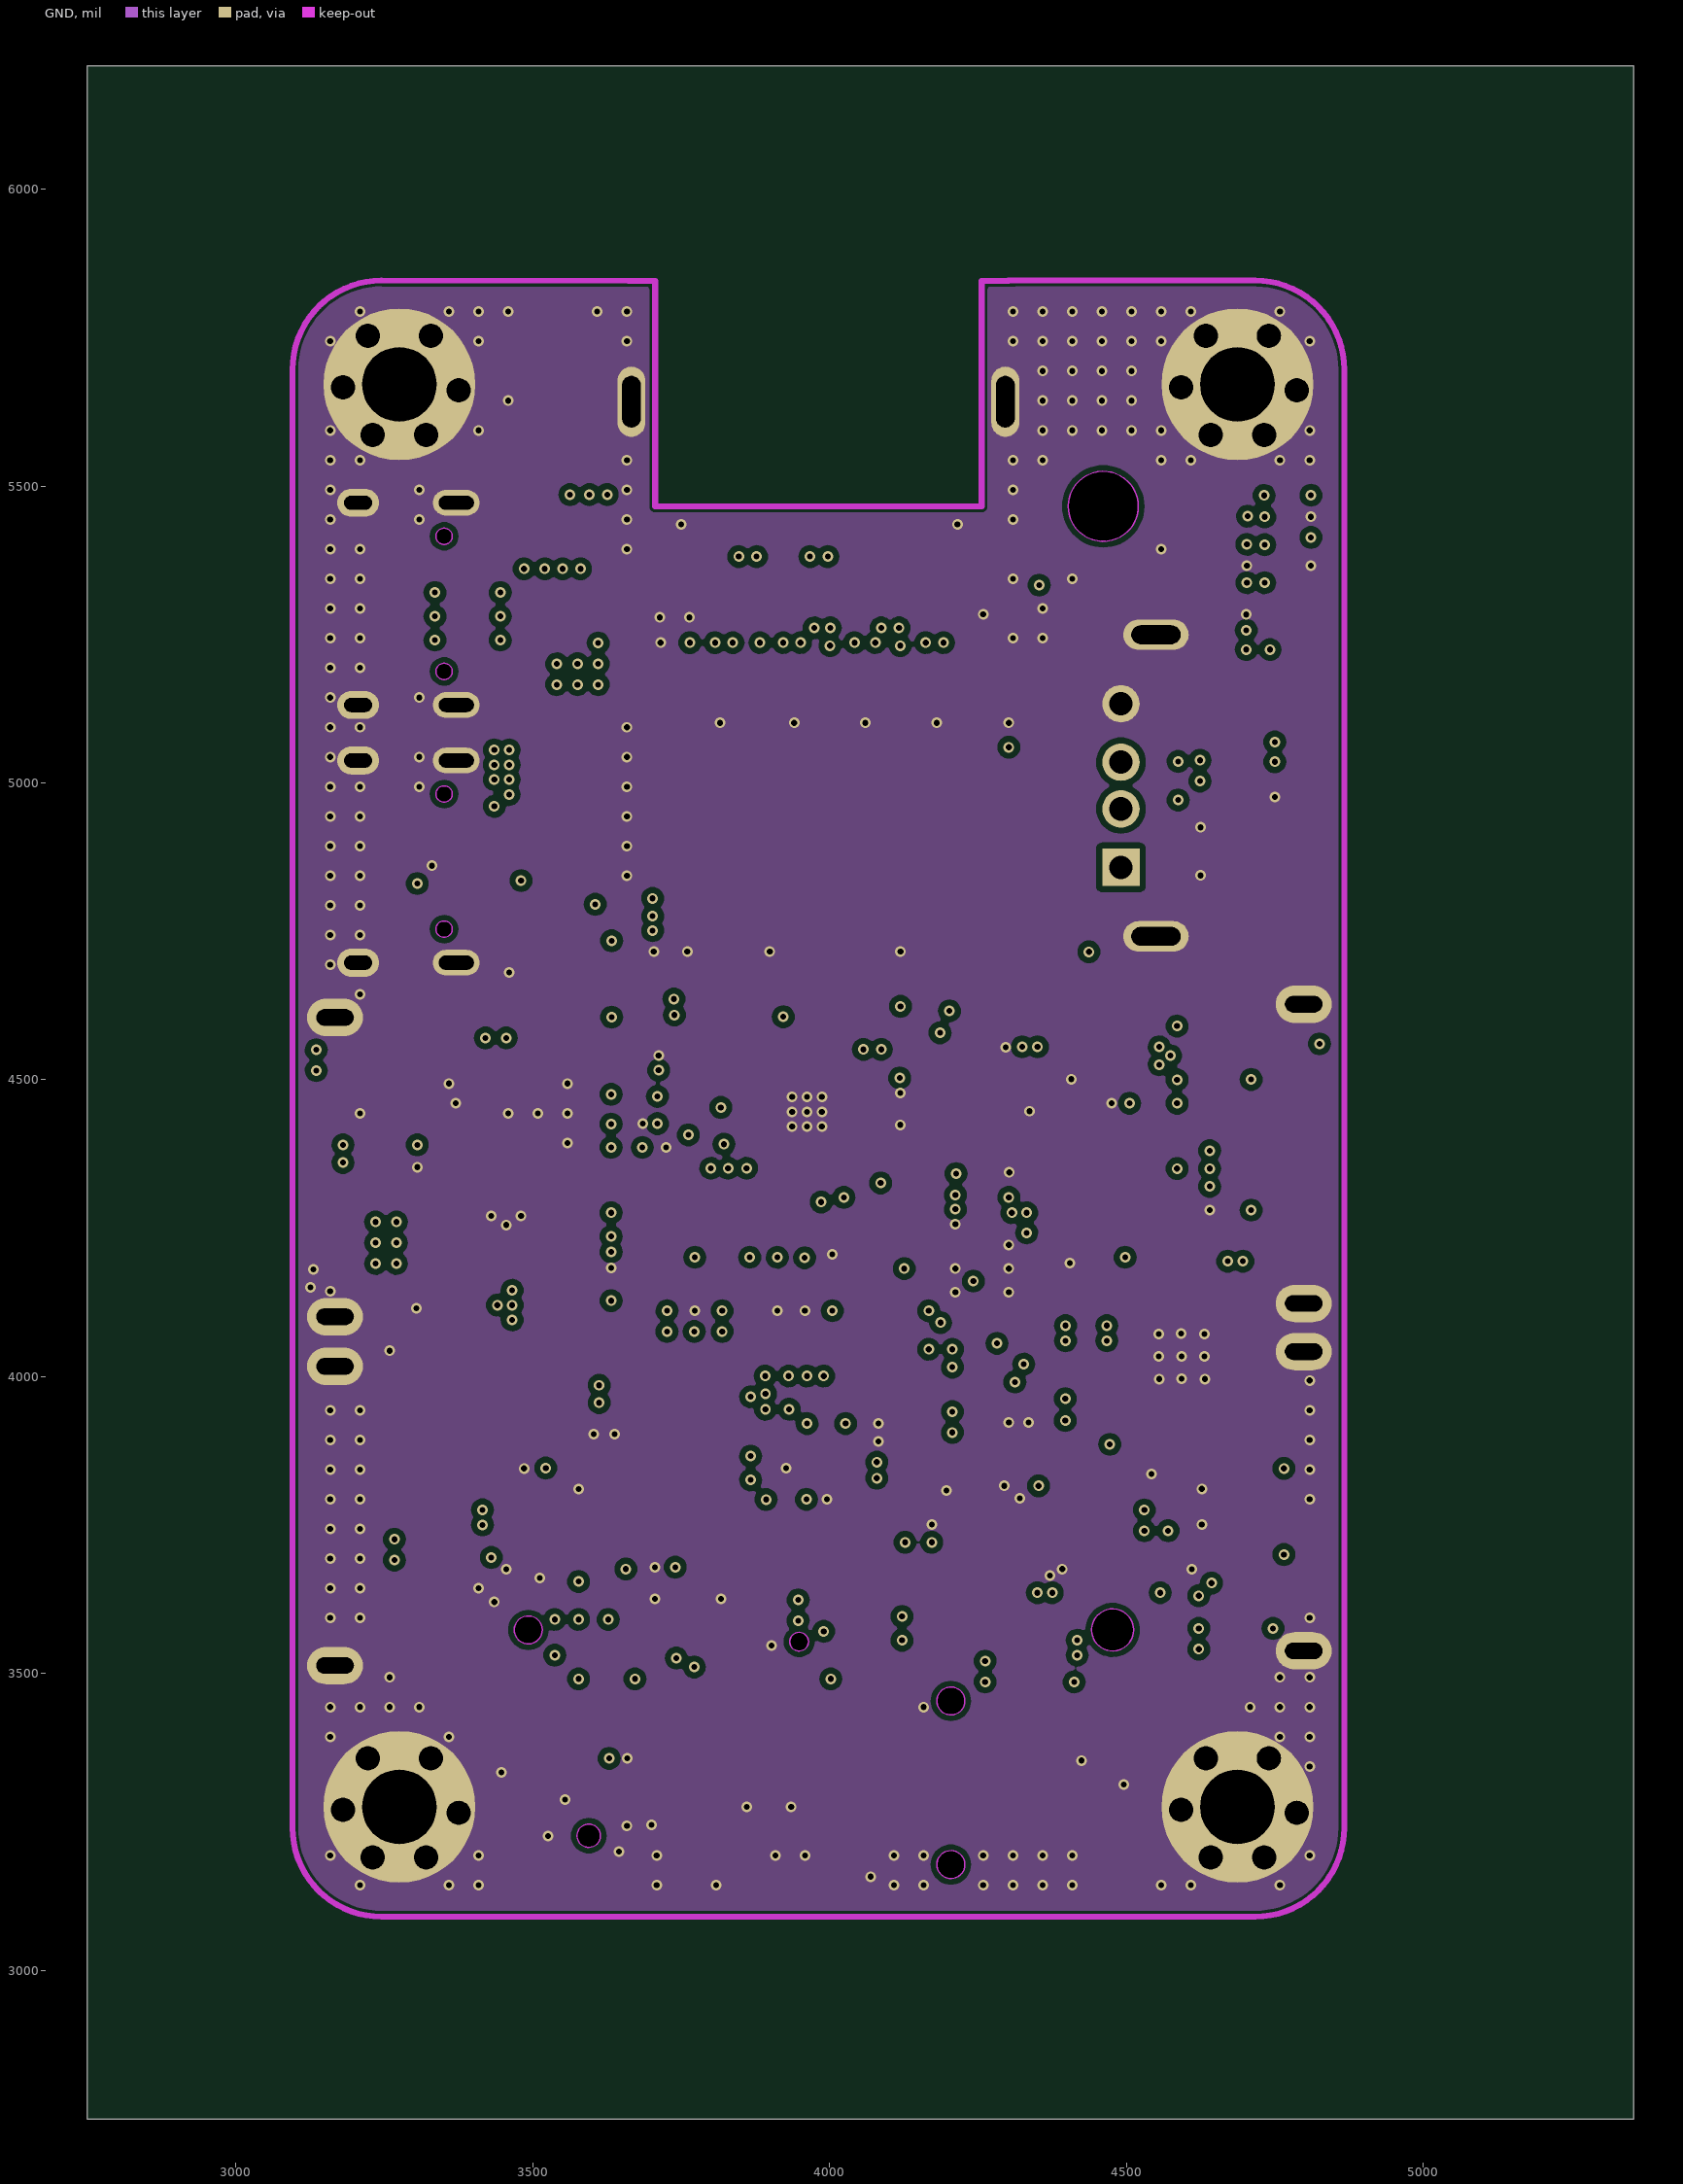
[diagram p0: GND]
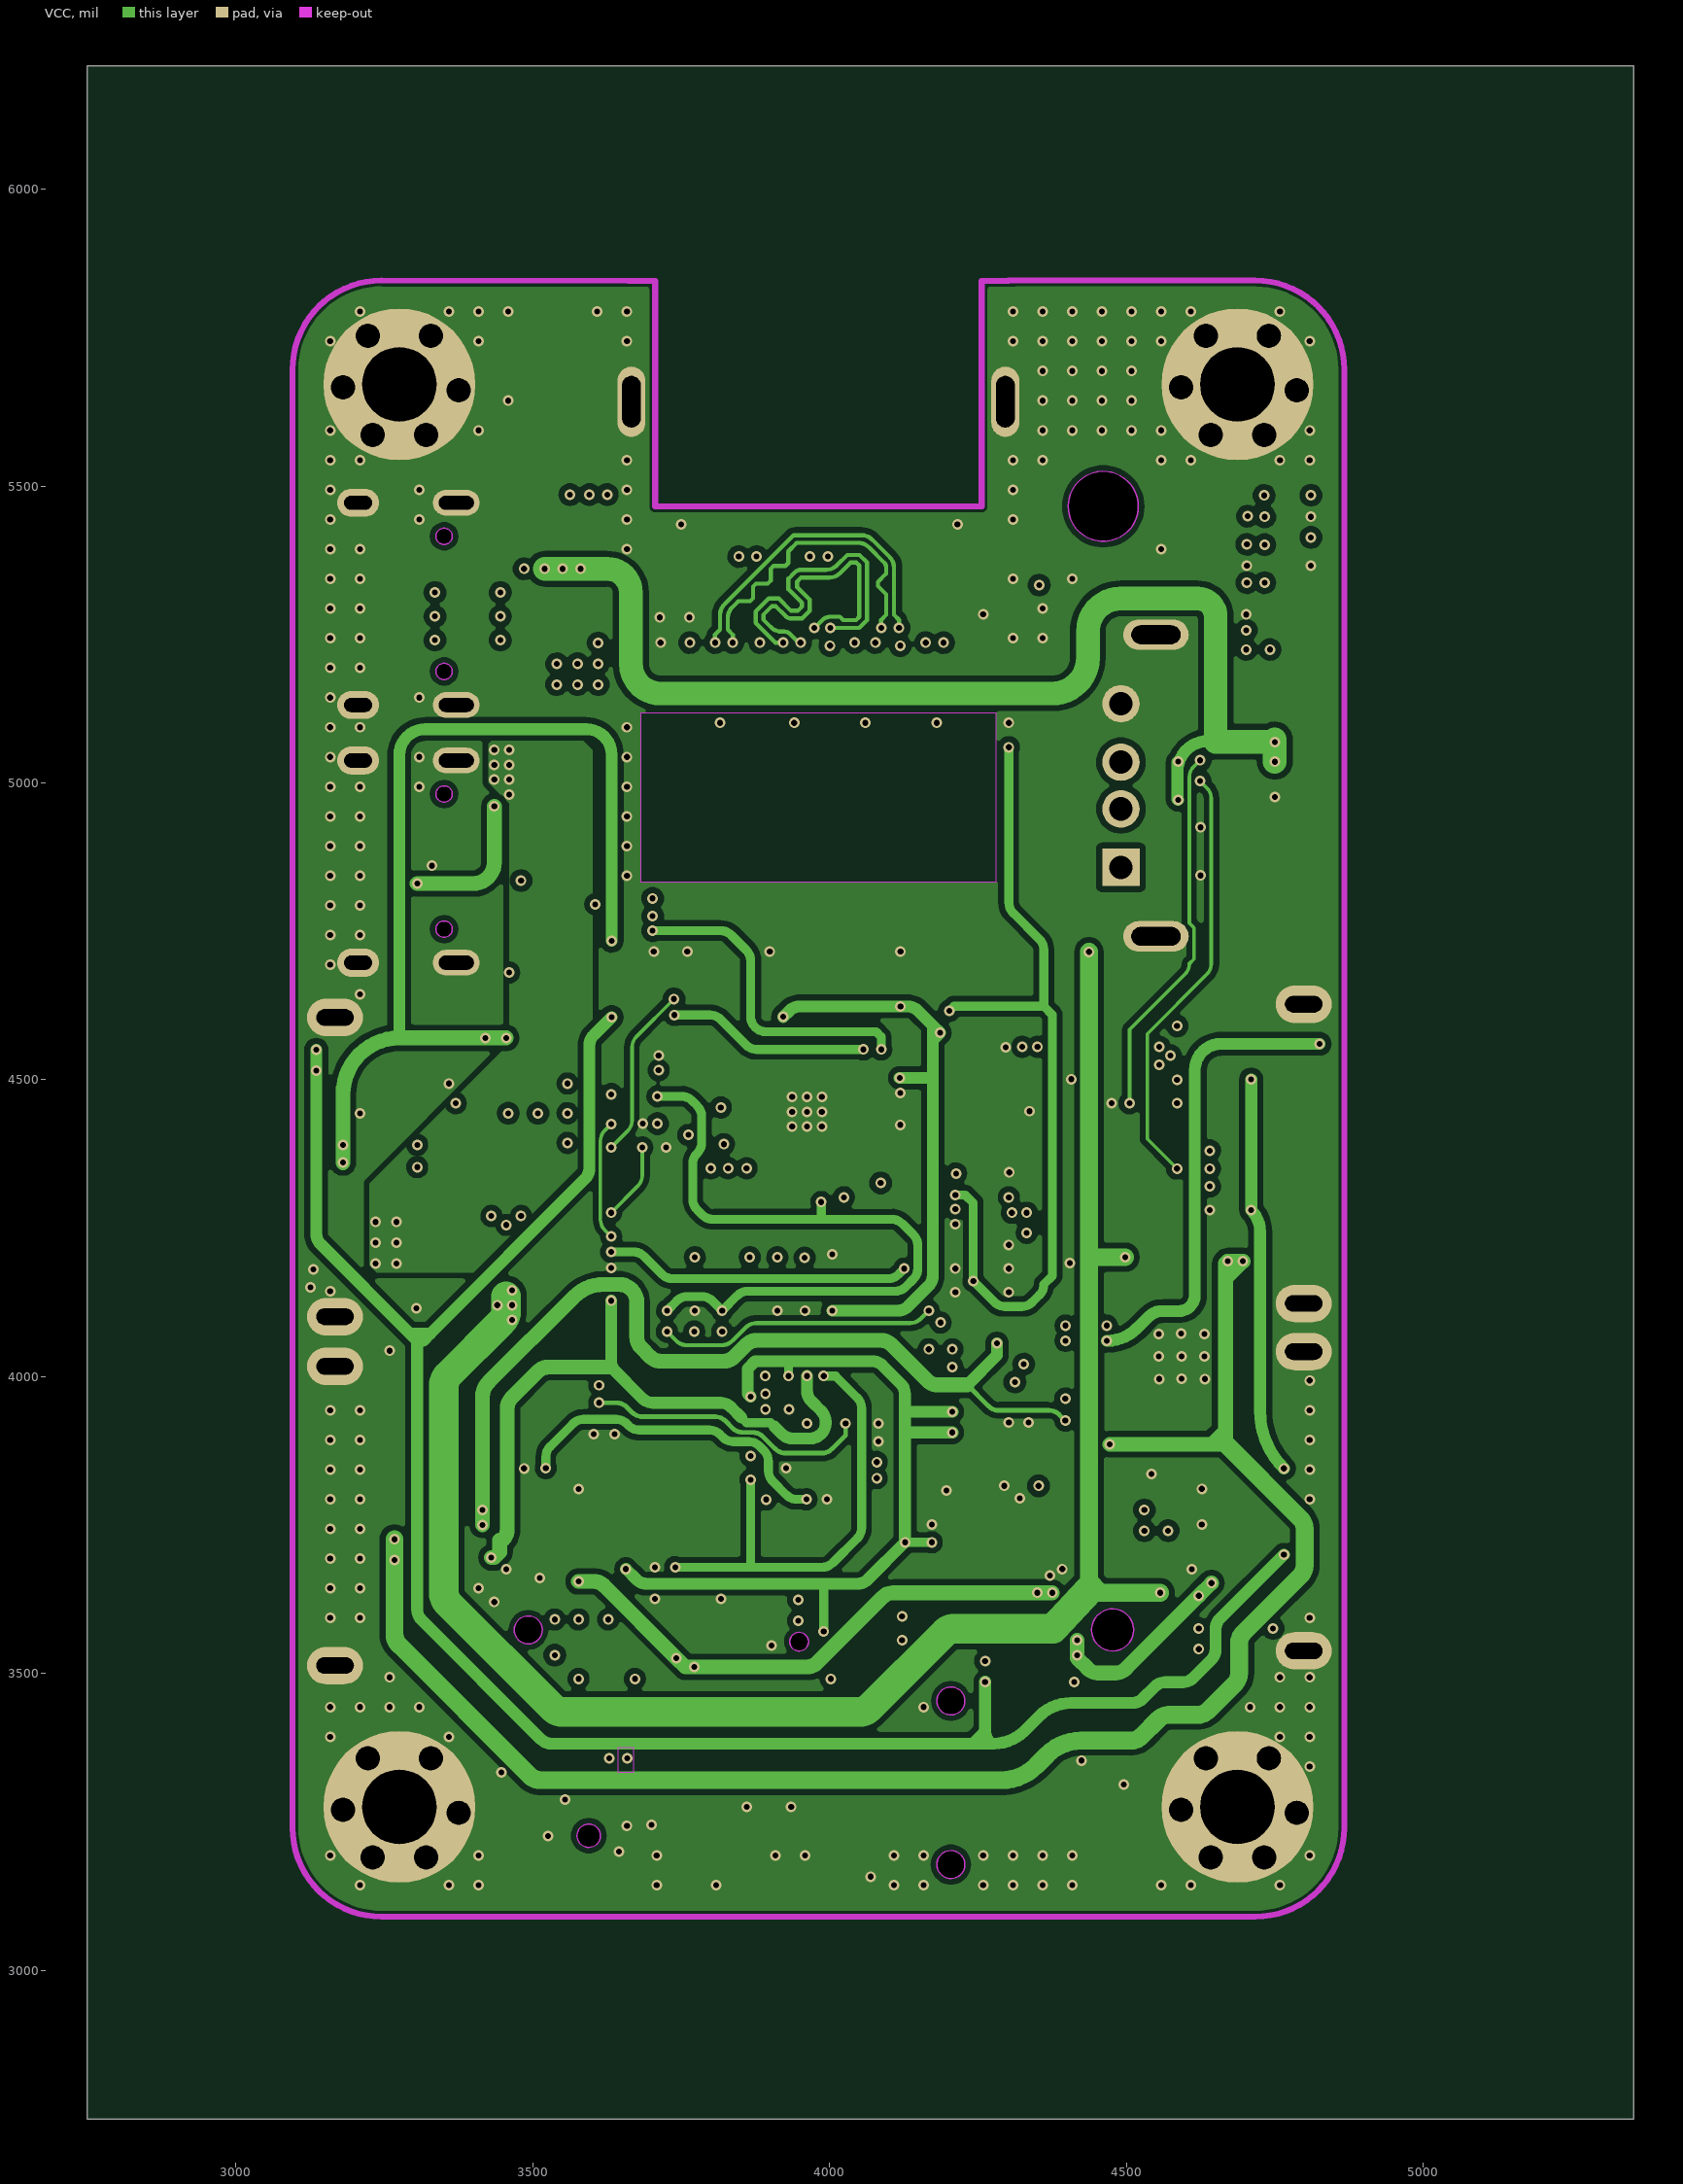
[diagram p1: VCC]
# Altium PCB MISC84334.PcbDoc (part 2 of 8)
## Components (designator, comment, footprint, x,y, rotation, side; value= is the part's Value field where it differs from the comment) (continued)
LED2 "XL-1005UGC" LED0402-RD_GREEN 3515.07,4020.59 r270 top
LED3 "XL-1005UGC" LED0402-RD_GREEN 3632.59,4337.09 r90 top
LED4 "XL-1005UGC" LED0402-RD_GREEN 3525.59,4805.59 r0 top
LED5 "XL-1005UGC" LED0402-RD_GREEN 4363.09,4992.53 r270 top
LED6 "XL-1005UGC" LED0402-RD_GREEN 4443.09,4010.59 r90 top
LED7 "XL-1005UGC" LED0402-RD_GREEN 4443.09,4133.09 r270 top
LED8 "19-217/GHC-YR1S2/3T" LED0603-RD 3595.59,3320.64 r180 bottom
Q1 "CJ2301 S1" SOT-23-3_L3.0-W1.7-P0.95-LS2.9-BR 3525.59,5280.59 r270 top
Q2 "MMBT5401" SOT-23-3_L2.9-W1.3-P1.90-LS2.4-BR 3525.59,5445.49 r270 top
Q3 "MMBT5401" SOT-23-3_L2.9-W1.3-P1.90-LS2.4-BR 3525.59,5605.59 r270 top
Q4 "SS8050" SOT-23-3_L2.9-W1.3-P1.90-LS2.4-BR 4650.59,4460.59 r270 bottom
Q5 "SS8050" SOT-23-3_L2.9-W1.3-P1.90-LS2.4-BR 4780.59,4460.59 r270 bottom
R1 "220kΩ" R0402 4568.63,3840.59 r270 bottom
R2 "15kΩ" R0402 4460.59,4148.54 r90 bottom
R3 "10kΩ" R0402 4415.59,4148.54 r270 bottom
R4 "50kΩ" R0402 4517.59,3840.59 r90 bottom
R5 "10kΩ" R0402 3475.59,5720.59 r270 top
R6 "50kΩ" R0402 3525.59,5720.59 r270 top
R7 "15kΩ" R0402 3605.59,4915.59 r270 bottom
R8 "232kΩ" R0402 3295.59,4915.59 r270 bottom
R9 "10kΩ" R0402 3605.59,4990.59 r270 bottom
R10 "4.7kΩ" R0402 3575.59,5720.59 r270 top
R11 "50kΩ" R0402 3395.59,4915.59 r90 bottom
R12 "10kΩ" R0603 3375.59,4390.59 r0 bottom
R13 "4.7kΩ" R0402 3865.8,4155.59 r90 top
R14 "4.7kΩ" R0402 4169.71,4222.09 r0 top
R15 "2.49kΩ" R0402 4169.59,4553.09 r0 top
R16 "4.7kΩ" R0402 3819.38,4155.59 r90 top
R17 "4.7kΩ" R0402 4169.65,4262.09 r0 top
R18 "4.7kΩ" R0402 3726.52,4155.59 r90 top
R19 "4.7kΩ" R0402 4169.77,4302.09 r0 top
R20 "4.7kΩ" R0402 3756.09,4456.33 r0 top
R21 "4.7kΩ" R0402 3756.09,4495.59 r0 top
R22 "4.7kΩ" R0402 3772.95,4155.59 r90 top
R23 "120Ω" R0402 4259.59,4345.09 r0 top
R24 "0Ω" R0402 3806.91,4665.59 r90 top
R25 "0Ω" R0402 3853.28,4665.59 r90 top
R26 "4.7kΩ" R0402 3958.66,4155.59 r90 top
R27 "0Ω" R0402 3946.02,4665.59 r90 top
R28 "100Ω" R0402 4169.9,4345.09 r0 top
R29 "0Ω" R0402 3992.38,4665.59 r90 top
R30 "4.7kΩ" R0402 3912.23,4155.59 r90 top
R31 "0Ω" R0402 4038.75,4665.59 r90 top
R32 "0Ω" R0402 4080.12,4665.59 r90 top
R33 "0Ω" R0402 4259.59,4262.09 r0 top
R34 "0Ω" R0402 4157.86,4665.59 r90 top
R35 "0Ω" R0402 4199.22,4665.59 r90 top
R36 "4.7kΩ" R0402 4259.59,4302.09 r0 top
R37 "75Ω" R0402 4120.59,5160.59 r90 bottom
R38 "75Ω" R0402 4000.59,5160.59 r90 bottom
R39 "75Ω" R0402 3880.59,5160.59 r90 bottom
R40 "75Ω" R0402 3765.59,5160.59 r90 bottom
R41 "22Ω" R0402 3958.66,4247.85 r270 top
R42 "10kΩ" R0402 3756.09,4578.09 r180 top
R43 "22Ω" R0402 3912.23,4247.85 r270 top
R44 "22Ω" R0402 3865.8,4247.85 r270 top
R45 "22Ω" R0402 3819.38,4247.85 r270 top
R46 "22Ω" R0402 3772.95,4247.85 r270 top
R47 "510Ω" R0402 3620.13,5395.59 r270 top
R48 "22Ω" R0402 3726.52,4247.85 r270 top
R49 "0Ω" R0402 3680.09,4247.85 r270 top
R50 "0Ω" R0402 4005.09,4155.59 r270 top
R51 "510Ω" R0402 4353.17,5395.59 r90 top
R52 "4.7kΩ" R0402 3565.22,4020.59 r270 top
R53 "4.7kΩ" R0402 3679.83,4338.09 r90 top
R54 "4.7kΩ" R0402 3525.59,4760.59 r0 top
R55 "4.7kΩ" R0402 4315.33,4993.09 r270 top
R56 "4.7kΩ" R0402 4397.83,4010.59 r90 top
R57 "4.7kΩ" R0402 4397.83,4133.09 r270 top
R58 "2.7kΩ" R0402 3893.29,3834.74 r90 bottom
R59 "100kΩ" R0402 4255.6,3751.19 r0 top
R60 "47kΩ" R0402 4335.95,3883.09 r0 top
R61 "100kΩ" R0402 4255.6,3838.09 r180 top
R62 "15kΩ" R0402 4020.73,3177.96 r180 top
R63 "0Ω" R0402 3477.77,3270.59 r270 top
R64 "0Ω" R0402 3478.09,3185.59 r270 top
R65 "0Ω" R0402 3478.04,3430.59 r90 top
R66 "4.7kΩ" R0402 4675.59,4330.59 r90 bottom
R67 "10kΩ" R0402 4650.59,4560.59 r0 bottom
R68 "2.2Ω" R0402 4035.29,3817.19 r0 bottom
R69 "2.2Ω" R0402 4035.29,3858.19 r0 bottom
R70 "10kΩ" R0402 3499.7,3321.19 r180 bottom
R71 "10kΩ" R0402 4780.59,4560.59 r180 bottom
R72 "4.7kΩ" R0402 4771.77,4330.59 r270 bottom
R73 "0Ω" R0402 4478.65,3335.59 r0 top
R74 "10kΩ" R0402 4478.65,3185.59 r180 top
R75 "1kΩ" R0402 4478.65,3285.59 r180 top
R76 "NC" R0805 3380.59,4075.59 r0 bottom
R77 "10kΩ" R0402 3325.59,3817.49 r180 bottom
R78 "10kΩ" R0402 3415.59,3816.03 r0 bottom
RJ1 "RC01812" RJ45-TH_RC01812 3981.44,5480.59 r0 top locked
U1 "MD7672B50SF4" ESOP-8_L4.9-W3.9-P1.27-LS6.0-BL-EP 4605.59,4035.59 r180 bottom
U2 "SY8113BADC" TSOT-23-6_L2.9-W1.6-P0.95-LS2.8-BR 3505.59,4895.59 r180 bottom
U3 "TP5108E23E-18" SOT-23-5_L3.0-W1.7-P0.95-LS2.8-BL 3370.59,4495.59 r270 bottom
U4 "RTL8211F-CG" WQFN-40_L5.0-W5.0-P0.4-BL-EP 3961.76,4445.59 r180 top
U5 "FE2.1-CQFP48A" LQFP-48_L7.0-W7.0-P0.50-LS9.0-BL 3980.59,3885.59 r180 top
U6 "SMTWE2050MTJ" SMD_BD4.4-L4.4-D2.8 4461.29,5465.79 r180 bottom
U7 "SY6280AAC" SOT-23-5_L3.0-W1.7-P0.95-LS2.8-BL 3370.59,3950.59 r270 bottom
USB1 "TYPE-C 16PIN 2MD(073)" USB-C-SMD_TYPE-C-6PIN-2MD-073 3299.59,5301.59 r270 top
USB2 "TYPE-C 16PIN 2MD(073)" USB-C-SMD_TYPE-C-6PIN-2MD-073 3299.59,4867.59 r270 top
USB4 "AF 10.0 HC6.3" USB-A-TH_AF-10.0-HC6.3 4520.59,4995.59 r90 top
X1 "25MHz" OSC-SMD_4P-L3.2-W2.5-BL 4257.09,4447.09 r270 top
X2 "12MHz" OSC-SMD_4P-L3.2-W2.5-BL 3647.73,3812.45 r90 top

## Footprints (in the part's own frame and the unit in brackets; to place one, negate y for a bottom-side part, rotate by r counter-clockwise, add the part's x,y. Pads: shape width x height; smd on the part's side, far side on the other; paste and mask are expansions set on the pad)
"125 X 300" [mil]
  round 40 hole 40 slot 40.2 at 0 deg paste+4 mask+4: 1(-95,-5) 1(100,-10)
  round 40 hole 40 slot 40.2 at 120 deg paste+4 mask+4: 1(-53,81.8) 1(45,-85)
  round 40 hole 40 slot 40.2 at 60 deg paste+4 mask+4: 1(-45,-85) 1(53,81.8)
  round 255.91 hole 125 slot 125.2 at 0 deg paste+4 mask+4: 1(0,0)
AUDIO-SMD_PJ-393 [mm]
  rect 2.5x1.4 smd: 1(3.45,-4) 2(3.45,-1.1) 3(3.45,1.8) 4(-3.45,2.1) 6(-3.45,-3) 7(-3.45,-0.1) 8(3.45,4)
  Board Outline Layer circle w0.003: c0,-4.5 r0.6
  Board Outline Layer circle w0.003: c0,2.5 r0.6
  Board Outline Layer region: 0.6,-4.5 0.54,-4.76 0.374,-4.969 0.133,-5.085 -0.134,-5.085 -0.374,-4.969 -0.541,-4.76 -0.6,-4.5 -0.6,-4.5 -0.541,-4.24 -0.374,-4.031 -0.134,-3.915 0.133,-3.915 0.374,-4.031 0.54,-4.24 0.6,-4.5
  Board Outline Layer region: 0.6,-4.5 0.591,-4.604 0.564,-4.705 0.519,-4.8 0.459,-4.886 0.386,-4.96 0.3,-5.02 0.205,-5.064 0.104,-5.091 0,-5.1 -0.104,-5.091 -0.205,-5.064 -0.3,-5.02 -0.386,-4.96 -0.46,-4.886 -0.52,-4.8 -0.564,-4.705 -0.591,-4.604 -0.6,-4.5 -0.591,-4.396 -0.564,-4.295 -0.52,-4.2 -0.46,-4.114 -0.386,-4.04 -0.3,-3.98 -0.205,-3.936 -0.104,-3.909 0,-3.9 0.104,-3.909 0.205,-3.936 0.3,-3.98 0.386,-4.04 0.459,-4.114 0.519,-4.2 0.564,-4.295 0.591,-4.396
  Board Outline Layer region: 0.6,2.5 0.54,2.239 0.374,2.031 0.133,1.915 -0.134,1.915 -0.374,2.031 -0.541,2.239 -0.6,2.5 -0.6,2.5 -0.541,2.76 -0.374,2.969 -0.134,3.085 0.133,3.085 0.374,2.969 0.54,2.76 0.6,2.5
  Board Outline Layer region: 0.6,2.5 0.591,2.396 0.564,2.295 0.519,2.2 0.459,2.114 0.386,2.04 0.3,1.98 0.205,1.936 0.104,1.909 0,1.9 -0.104,1.909 -0.205,1.936 -0.3,1.98 -0.386,2.04 -0.46,2.114 -0.52,2.2 -0.564,2.295 -0.591,2.396 -0.6,2.5 -0.591,2.604 -0.564,2.705 -0.52,2.8 -0.46,2.885 -0.386,2.959 -0.3,3.019 -0.205,3.064 -0.104,3.091 0,3.1 0.104,3.091 0.205,3.064 0.3,3.019 0.386,2.959 0.459,2.885 0.519,2.8 0.564,2.705 0.591,2.604
  Multi-Layer board cut-out: 0.6,-4.5 0.54,-4.76 0.374,-4.969 0.133,-5.085 -0.134,-5.085 -0.374,-4.969 -0.541,-4.76 -0.6,-4.5 -0.6,-4.5 -0.541,-4.24 -0.374,-4.031 -0.134,-3.915 0.133,-3.915 0.374,-4.031 0.54,-4.24 0.6,-4.5
  Multi-Layer board cut-out: 0.6,2.5 0.54,2.239 0.374,2.031 0.133,1.915 -0.134,1.915 -0.374,2.031 -0.541,2.239 -0.6,2.5 -0.6,2.5 -0.541,2.76 -0.374,2.969 -0.134,3.085 0.133,3.085 0.374,2.969 0.54,2.76 0.6,2.5
  silkscreen extent -3,-8 3.9,6.5
C0603 [mm]
  rect 0.8x0.9 smd paste+0 mask+0.051: 1(-0.7,0) 2(0.7,0)
D0402-BI [mm]
  rect 0.6x0.6 smd paste-100 mask+0.051: 1(-0.5,0) 2(0.5,0)
  silkscreen extent -0.11,-0.25 0.1,0.25
ESOP-8_L4.9-W3.9-P1.27-LS6.0-BL-EP [mm]
  rect 0.6x1.2 smd: 1(-1.905,-2.908) 2(-0.635,-2.908) 3(0.635,-2.908) 4(1.905,-2.908) 5(1.905,2.908) 6(0.635,2.908) 7(-0.635,2.908) 8(-1.905,2.908)
  rect 3.3x2.4 smd: 9(0,0)
  silkscreen extent -3.2,-2.67 2.55,2.05
F0805 [mm]
  rect 1.335x1.5 smd paste-100 mask+0.051: 1(-1.142,0) 2(1.142,0)
  silkscreen extent -0.19,-0.38 0.19,0.38
fpc-smd_p0.30-39p_fgs-xj-h1.0 [mm]
  rect 0.3x0.65 smd paste+0 mask+0.051: 1(5.7,-1.55) 2(5.4,1.55) 3(5.1,-1.55) 4(4.8,1.55) 5(4.5,-1.55) 6(4.2,1.55) 7(3.9,-1.55) 8(3.6,1.55) 9(3.3,-1.55) 10(3,1.55) 11(2.7,-1.55) 12(2.4,1.55) 13(2.1,-1.55) 14(1.8,1.55) 15(1.5,-1.55) 16(1.2,1.55) 17(0.9,-1.55) 18(0.6,1.55) 19(0.3,-1.55) 20(0,1.55) 21(-0.3,-1.55) 22(-0.6,1.55) 23(-0.9,-1.55) 24(-1.2,1.55) 25(-1.5,-1.55) 26(-1.8,1.55) 27(-2.1,-1.55) 28(-2.4,1.55) 29(-2.7,-1.55) 30(-3,1.55) 31(-3.3,-1.55) 32(-3.6,1.55) 33(-3.9,-1.55) 34(-4.2,1.55) 35(-4.5,-1.55) 36(-4.8,1.55) 37(-5.1,-1.55) 38(-5.4,1.55) 39(-5.7,-1.55)
  rect 0.4x0.95 smd paste+0 mask+0.051: 40(-6.35,-1.2) 41(6.35,-1.2)
  silkscreen extent -6.71,-2.37 6.7,1.55
IND-SMD_L2.5-W2.0_WPN252012H [mm]
  rect 1.724x1.87 smd: 1(1.228,0) 2(-1.228,0)
L0603 [mm]
  rect 0.8x0.864 smd paste-100 mask+0.051: 1(-0.7,0) 2(0.7,0)
LED0402-RD_GREEN [mm]
  rect 0.636x0.54 smd paste-100 mask+0.051: 1(-0.538,0) 2(0.538,0)
  silkscreen extent -1.12,-0.35 -0.97,0.35
LED0603-RD [mm]
  rect 0.8x0.8 smd: 1(-0.85,-0.01) 2(0.749,-0.003)
  silkscreen extent -0.17,-0.33 0.17,0.35
LQFP-48_L7.0-W7.0-P0.50-LS9.0-BL [mm]
  oval 0.27x1.5 smd paste+0 mask+0.05: 1(-2.75,-4.25) 2(-2.25,-4.25) 3(-1.75,-4.25) 4(-1.25,-4.25) 5(-0.75,-4.25) 6(-0.25,-4.25) 7(0.25,-4.25) 8(0.75,-4.25) 9(1.25,-4.25) 10(1.75,-4.25) 11(2.25,-4.25) 12(2.75,-4.25) 25(2.75,4.25) 26(2.25,4.25) 27(1.75,4.25) 28(1.25,4.25) 29(0.75,4.25) 30(0.25,4.25) 31(-0.25,4.25) 32(-0.75,4.25) 33(-1.25,4.25) 34(-1.75,4.25) 35(-2.25,4.25) 36(-2.75,4.25)
  oval 1.5x0.27 smd paste+0 mask+0.05: 13(4.25,-2.75) 14(4.25,-2.25) 15(4.25,-1.75) 16(4.25,-1.25) 17(4.25,-0.75) 18(4.25,-0.25) 19(4.25,0.25) 20(4.25,0.75) 21(4.25,1.25) 22(4.25,1.75) 23(4.25,2.25) 24(4.25,2.75) 37(-4.25,2.75) 38(-4.25,2.25) 39(-4.25,1.75) 40(-4.25,1.25) 41(-4.25,0.75) 42(-4.25,0.25) 43(-4.25,-0.25) 44(-4.25,-0.75) 45(-4.25,-1.25) 46(-4.25,-1.75) 47(-4.25,-2.25) 48(-4.25,-2.75)
  silkscreen extent -3.59,-4.46 3.3,3.34
OSC-SMD_4P-L3.2-W2.5-BL [mm]
  rect 1.4x1.2 smd: 1(-1.1,-0.875) 2(1.1,-0.875) 3(1.1,0.875) 4(-1.1,0.875)
  silkscreen extent -2.07,-1.75 -1.56,-1.24